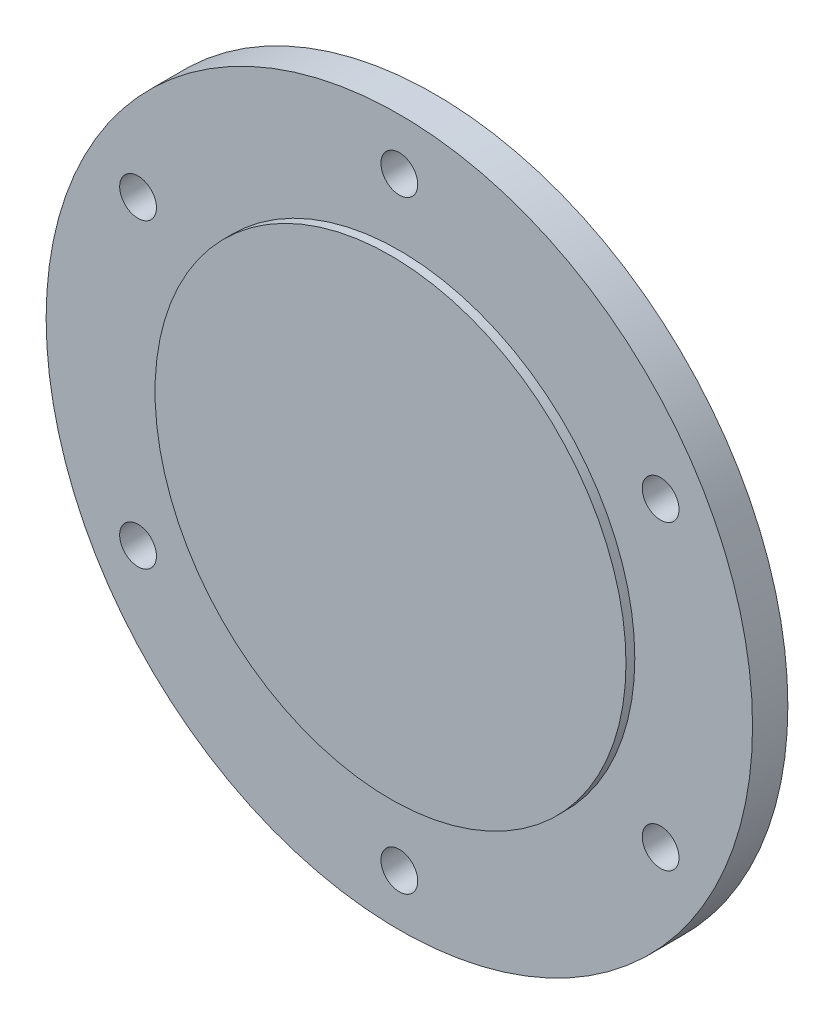
SolidWorks part; units mm, degrees
ref_plane "Front Plane" through (0, 0, 0) normal (0, 0, 1) x (1, 0, 0)
ref_plane "Top Plane" through (0, 0, 0) normal (0, 1, 0) x (1, 0, 0)
ref_plane "Right Plane" through (0, 0, 0) normal (1, 0, 0) x (0, 0, -1)
ref_plane "Plane1" through (0, 234.744, 0) normal (0, 1, 0) x (1, 0, 0)
sketch "Sketch1" plane through (0, 234.744, 0) normal (0, 1, 0) x (1, 0, 0)
  line L0 (641.2306, 150.693) -> (521.2306, 150.693)
  line L1 (521.2306, 150.693) -> (521.2306, 138.693)
  line L2 (521.2306, 138.693) -> (641.2306, 138.693)
  line L3 (641.2306, 138.693) -> (641.2306, 150.693)
  line L4 (521.2306, 150.693) -> (521.2306, 138.693) construction
  dimension "D1" = 120
  dimension "D2" = 12
revolve "Revolve1" add sketch "Sketch1" angle 360 about L4
sketch "Sketch2" plane through (0, 0, -150.693) normal (0, 0, -1) x (-1, 0, 0)
  circle A0 centre (-521.2306, 234.744) radius 85
  dimension "D1" = 170
extrude "Boss-Extrude1" add sketch "Sketch2" along normal blind 2.5
sketch "Sketch3" plane through (0, 0, -138.693) normal (0, 0, 1) x (1, 0, 0)
  circle A0 centre (521.2306, 234.744) radius 80
  dimension "D1" = 160
extrude "Boss-Extrude2" add sketch "Sketch3" along normal blind 3
hole_wizard "Ø12.5 (12.5) Diameter Hole1" positions "Sketch5" profile "Sketch4" hole size "Ø12.5" standard "ANSI Metric"
sketch "Sketch5" plane through (0, 0, -138.693) normal (0, 0, 1) x (1, 0, 0)
  point P0 (521.2306, 337.244)
  point P1 (609.9982, 285.994)
  point P2 (432.463, 285.994)
  point P3 (432.463, 183.494)
  point P4 (521.2306, 132.244)
  point P5 (609.9982, 183.494)
sketch "Sketch4" plane through (521.2306, 337.244, -138.693) normal (1, 0, 0) x (0, -1, 0)
  line L0 (0, 0) -> (0, 14.5)
  line L1 (0, 14.5) -> (6.25, 14.5)
  line L2 (6.25, 14.5) -> (6.25, 0)
  line L5 (6.25, 0) -> (0, 0)
  line L11 (0, -6.35) -> (0, 107.95) construction
  dimension "通孔孔直径" = 12.5
  dimension "通孔孔深度" = 14.5
hole_wizard "M90 counterbore hole1" positions "Sketch7" profile "Sketch6" counterbore size "M90" standard "ANSI Metric"
sketch "Sketch7" plane through (0, 0, -153.193) normal (0, 0, -1) x (-1, 0, 0)
  point P0 (-521.2306, 234.744)
sketch "Sketch6" plane through (521.2306, 234.744, -153.193) normal (1, 0, 0) x (0, 1, 0)
  line L0 (0, 0) -> (0, 17.5)
  line L1 (0, 17.5) -> (50, 17.5)
  line L3 (50, 17.5) -> (50, 1)
  line L4 (50, 1) -> (65, 1)
  line L5 (65, 1) -> (65, 0)
  line L7 (65, 0) -> (0, 0)
  line L11 (0, -6.35) -> (0, 107.95) construction
  dimension "通孔孔直径" = 100
  dimension "通孔孔深度" = 17.5
  dimension "柱形沉头孔直径" = 130
  dimension "柱形沉头孔深度" = 1
sketch "Sketch8" plane through (0, 0, -135.693) normal (0, 0, 1) x (1, 0, 0)
  circle A0 centre (521.2306, 234.744) radius 50.1019
extrude "Boss-Extrude3" add sketch "Sketch8" against normal blind 7
